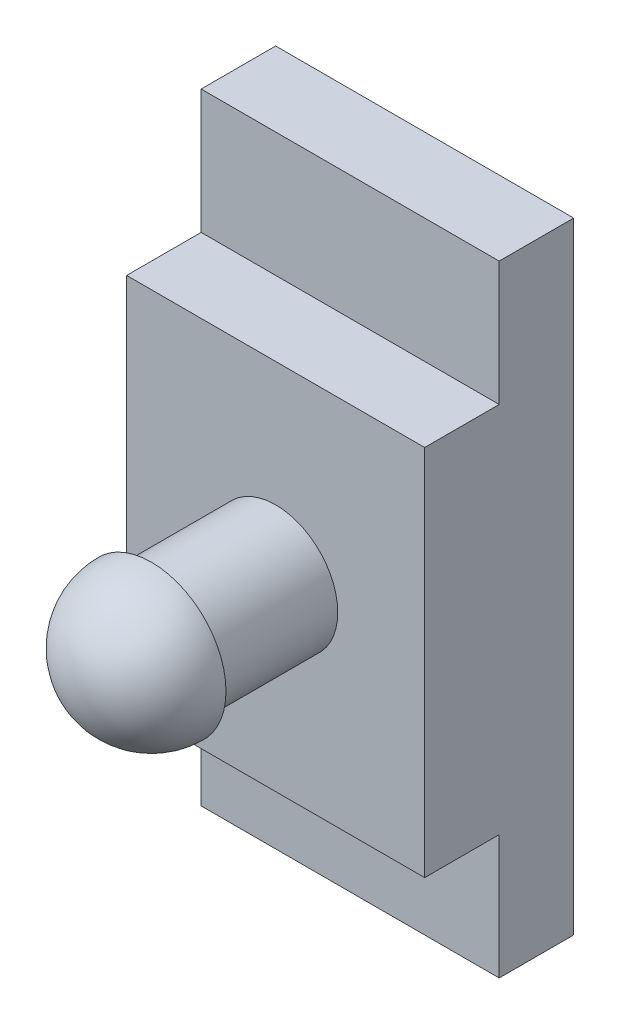
from build123d import *

# Parameters (mm, degrees)
SKETCH1_W           = 12
SKETCH1_H           = 25
BOSS_EXTRUDE1_DEPTH = 3
SKETCH2_W           = 12
SKETCH2_H           = 15
BOSS_EXTRUDE2_DEPTH = 3
SKETCH3_R           = 2.5
BOSS_EXTRUDE3_DEPTH = 5
SCALE1_SCALE        = 2.5


with BuildPart() as part:
    # Sketch1 → Boss-Extrude1 (new body)
    with BuildSketch(Plane.XY):
        Rectangle(SKETCH1_W, SKETCH1_H)
    extrude(amount=BOSS_EXTRUDE1_DEPTH)

    # Sketch2 → Boss-Extrude2 (add)
    with BuildSketch(Plane.XY.offset(3)):
        Rectangle(SKETCH2_W, SKETCH2_H)
    extrude(amount=BOSS_EXTRUDE2_DEPTH)

    # Sketch3 → Boss-Extrude3 (add)
    with BuildSketch(Plane.XY.offset(6)):
        Circle(SKETCH3_R)
    extrude(amount=BOSS_EXTRUDE3_DEPTH)

    # Sketch4 → Revolve1 (revolve)
    with BuildSketch(Plane(origin=(0, 0, 0), x_dir=(1, 0, 0), z_dir=(0, 1, 0))):
        with BuildLine():
            Line((0, -11), (3, -11))
            ThreePointArc((3, -11), (2.121320344, -13.121320344), (0, -14))
            Line((0, -14), (0, -11))
        make_face()
    revolve(axis=Axis((0, 0, 11), (0, 0, 1)))


with BuildPart() as part_1:
    # Scale1: scaled about (0, 0, 0)
    add(part.part.scale(SCALE1_SCALE))


solid = part_1.part
